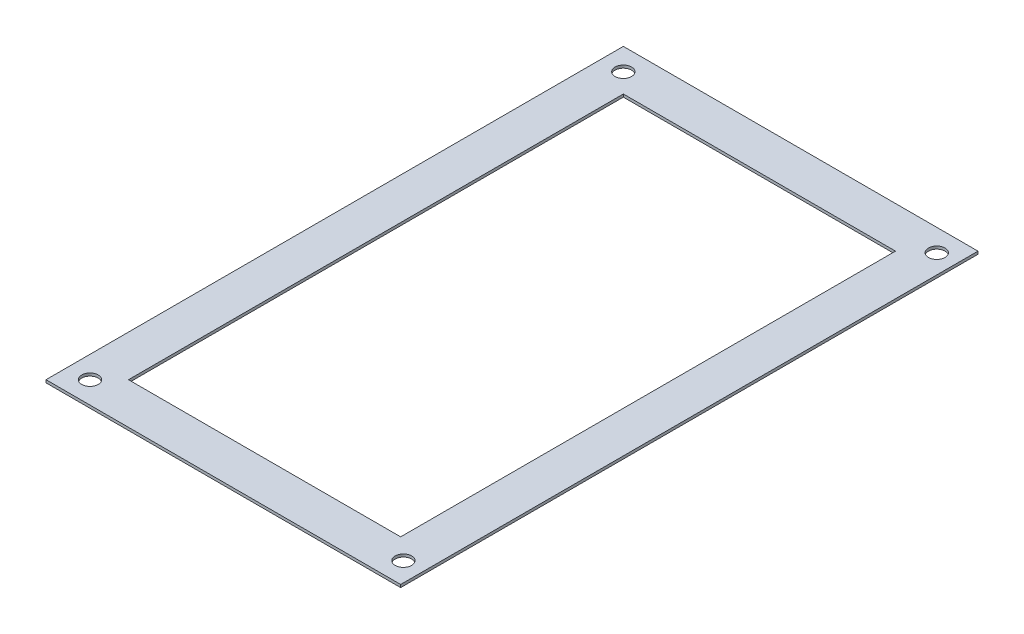
SolidWorks part; units mm, degrees
ref_plane "Front" through (0, 0, 0) normal (0, 0, 1) x (1, 0, 0)
ref_plane "Top" through (0, 0, 0) normal (0, 1, 0) x (1, 0, 0)
ref_plane "Right" through (0, 0, 0) normal (1, 0, 0) x (0, 0, -1)
sketch "Sketch1" plane through (0, 0, 0) normal (0, 1, 0) x (1, 0, 0)
  line L0 (-25.5961, 15) -> (-25.5961, 195)
  line L1 (-40.5961, 0) -> (88.4039, 0)
  line L2 (-40.5961, 0) -> (-40.5961, 210)
  line L3 (-40.5961, 210) -> (88.4039, 210)
  line L4 (88.4039, 0) -> (88.4039, 210)
  line L5 (-25.5961, 195) -> (73.4039, 195)
  line L6 (73.4039, 15) -> (73.4039, 195)
  line L7 (-25.5961, 15) -> (73.4039, 15)
  line L8 (-73.758, 202) -> (103.5079, 202) construction
  line L9 (81.4039, 225.4398) -> (81.4039, -26.9129) construction
  line L10 (-73.758, 8) -> (192.0508, 8) construction
  line L11 (-32.5961, 225.4398) -> (-32.5961, -15.8032) construction
  circle A0 centre (-32.5961, 8) radius 3
  circle A1 centre (81.4039, 8) radius 3
  circle A2 centre (81.4039, 202) radius 3
  circle A3 centre (-32.5961, 202) radius 3
  dimension "D7" = 6
  dimension "D8" = 6
  dimension "D9" = 6
  dimension "D10" = 6
  dimension "D1" = 210
  dimension "D2" = 129
  dimension "D4" = 8
  dimension "D5" = 8
  dimension "D6" = 8
  dimension "D11" = 114
  dimension "D3" = 15
extrude "Boss-Extrude1" add sketch "Sketch1" along normal blind 1
scale "Scale 1" bodies to scale 101 scale about centroid uniform scaling yes scale factor 1.875
